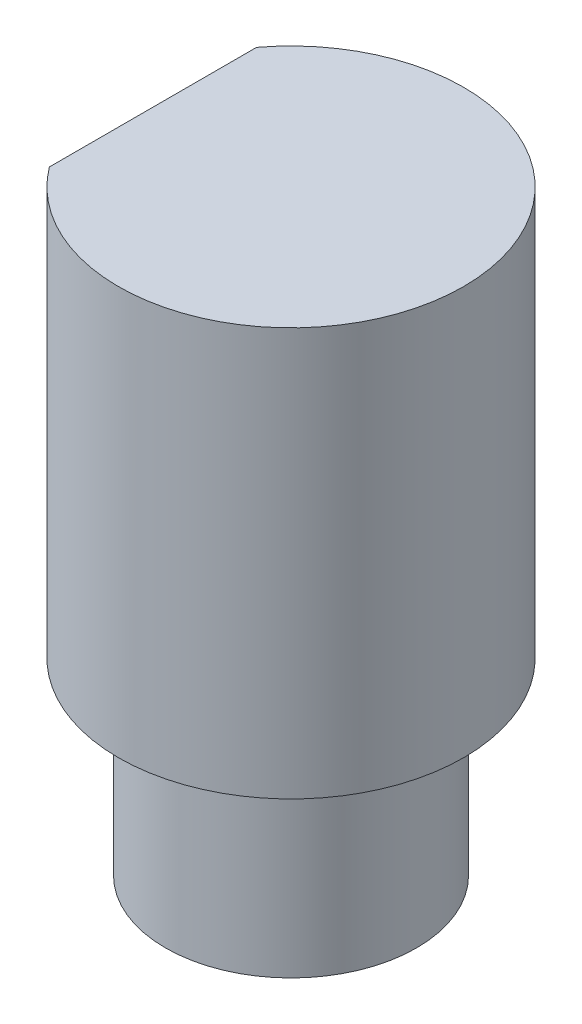
SolidWorks part; units mm, degrees
ref_plane "Front Plane" through (0, 0, 0) normal (0, 0, 1) x (1, 0, 0)
ref_plane "Top Plane" through (0, 0, 0) normal (0, 1, 0) x (1, 0, 0)
ref_plane "Right Plane" through (0, 0, 0) normal (1, 0, 0) x (0, 0, -1)
sketch "Sketch1" plane through (0, 0, 0) normal (0, 1, 0) x (1, 0, 0)
  circle A0 centre (0, 0) radius 20
  dimension "D1" = 40
extrude "Boss-Extrude1" add sketch "Sketch1" along normal blind 30
sketch "Sketch2" plane through (0, 30, 0) normal (0, 1, 0) x (1, 0, 0)
  circle A0 centre (0, 0) radius 27.5
  dimension "D1" = 55
extrude "Boss-Extrude2" add sketch "Sketch2" along normal blind 65
sketch "Sketch3" plane through (0, 0, 0) normal (1, 0, 0) x (0, 0, -1)
  line L0 (27.5, 95) -> (-27.5, 95) construction
  line L1 (-17.5, 95) -> (17.5, 95)
  line L2 (-17.5, 95) -> (-17.5, 40)
  line L3 (-17.5, 40) -> (17.5, 40)
  line L4 (17.5, 95) -> (17.5, 40)
  line L5 (-27.5, 95) -> (-27.5, 30) construction
  line L6 (27.5, 30) -> (27.5, 95) construction
  dimension "D1" = 55
  dimension "D2" = 10
  dimension "D3" = 10
extrude "Cut-Extrude1" cut sketch "Sketch3" against normal blind 65 from offset 22 offset against normal yes
sketch "Sketch4" plane through (-22, 0, 0) normal (-1, 0, 0) x (0, 0, 1)
  line L0 (16.5, 95) -> (-16.5, 95) construction
  circle A0 centre (0, 73) radius 11.3
  dimension "D1" = 22.6
  dimension "D2" = 22
extrude "Cut-Extrude2" cut sketch "Sketch4" against normal blind 40
sketch "Sketch5" plane through (0, 0, 0) normal (0, -1, 0) x (1, 0, 0)
  circle A0 centre (0, 0) radius 9.3
  dimension "D1" = 18.6
extrude "Cut-Extrude3" cut sketch "Sketch5" against normal blind 74
